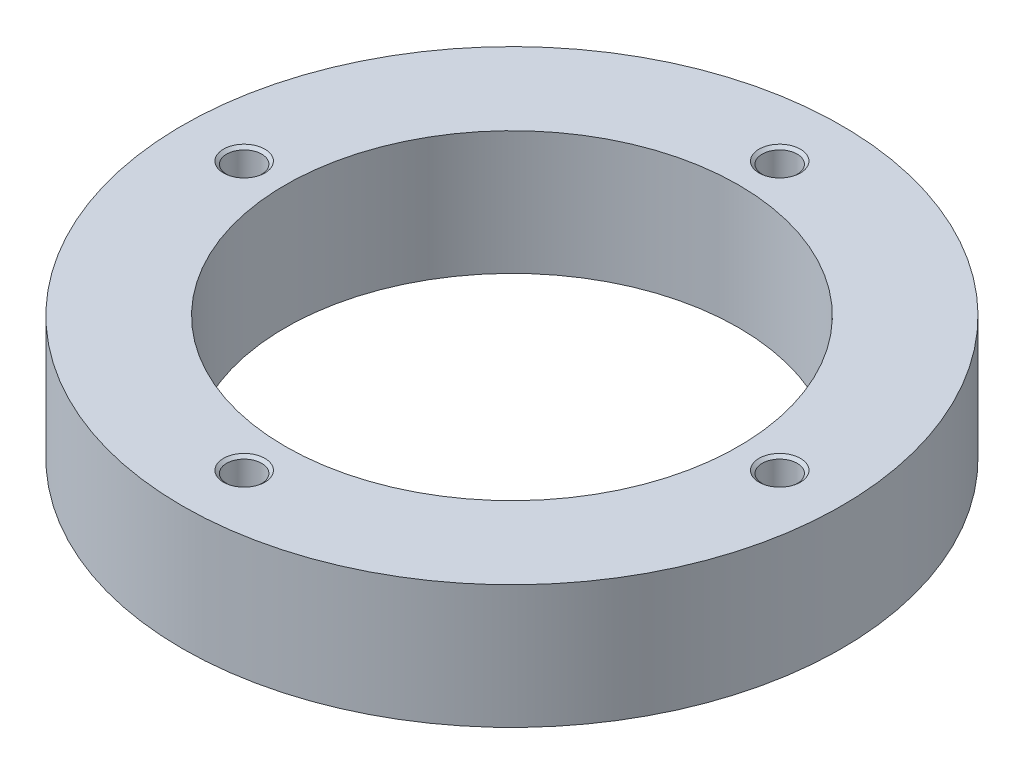
SolidWorks part; units mm, degrees
ref_plane "Front Plane" through (0, 0, 0) normal (0, 0, 1) x (1, 0, 0)
ref_plane "Top Plane" through (0, 0, 0) normal (0, 1, 0) x (1, 0, 0)
ref_plane "Right Plane" through (0, 0, 0) normal (1, 0, 0) x (0, 0, -1)
sketch "Sketch1" plane through (0, 0, 0) normal (0, 1, 0) x (1, 0, 0)
  line L0 (-107.9412, 0) -> (106.532, 0) construction
  line L2 (0, 91.8768) -> (0, -94.4133) construction
  circle A0 centre (0, 0) radius 80
  circle A1 centre (0, 0) radius 65 construction
  circle A2 centre (0, 0) radius 55
  dimension "D1" = 160
  dimension "D2" = 110
  dimension "130" = 130
extrude "Boss-Extrude1" add sketch "Sketch1" along normal blind 30
hole_wizard "M10 Tapped Hole1" positions "Sketch4" profile "Sketch5" tap size "M10" standard "GB"
sketch "Sketch4" plane through (0, 30, 0) normal (0, 1, 0) x (1, 0, 0)
  line L0 (0, 0) -> (80, 0) construction
  line L1 (0, 0) -> (0, 80) construction
  circle A0 centre (0, 0) radius 65 construction
  circle A1 centre (0, 0) radius 80 construction
  point P22 (65, 0)
  point P31 (0, -65)
  point P32 (-65, 0)
  point P33 (0, 65)
  dimension "D1" = 130
  dimension "D2" = 4
sketch "Sketch5" plane through (0, 30, -65) normal (1, 0, 0) x (0, 0, 1)
  line L0 (0, 0) -> (0, 24.5537)
  line L1 (0, 24.5537) -> (4.25, 22)
  line L2 (4.25, 22) -> (4.25, 0.6503)
  line L3 (4.25, 0.6503) -> (5.025, 0)
  line L5 (5.025, 0) -> (0, 0)
  line L6 (-4.25, 0.6503) -> (-5.025, 0) construction
  line L10 (0, 24.5537) -> (-4.25, 22) construction
  line L11 (0, -6.35) -> (0, 107.95) construction
  dimension "螺纹孔钻头直径" = 8.5
  dimension "螺纹孔钻头深度" = 22
  dimension "近端锥形沉头孔直径" = 10.05
  dimension "近端锥形沉头孔角度" = 100
  dimension "导头角度" = 118
cosmetic thread "Cosmetic thread 1"
cosmetic thread "Cosmetic thread 2"
cosmetic thread "Cosmetic thread 3"
cosmetic thread "Cosmetic thread 4"
